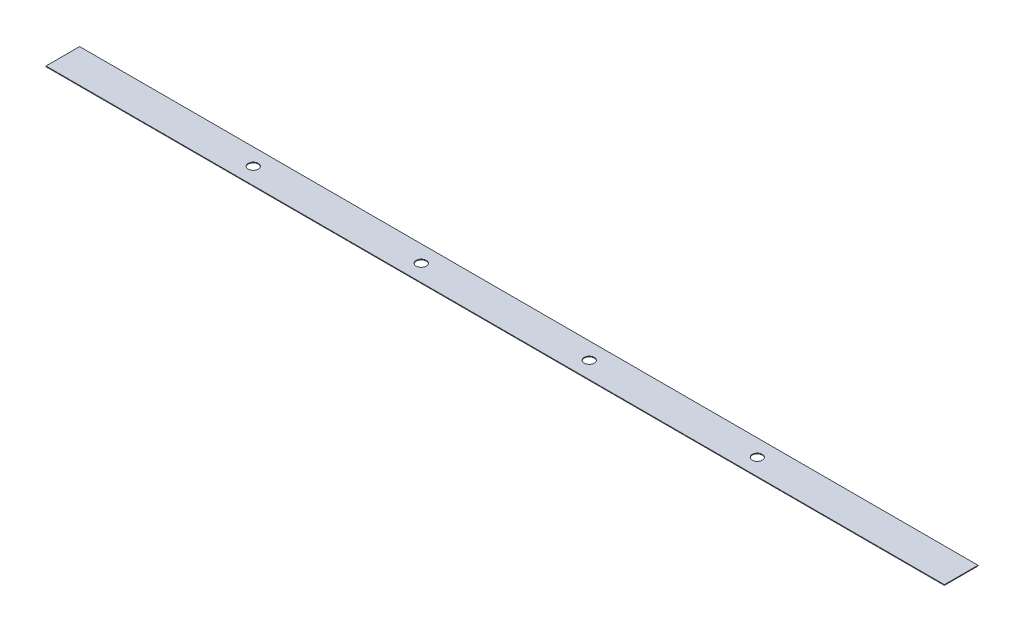
SolidWorks part; units mm, degrees
material "45"
ref_plane "Front Plane" through (0, 0, 0) normal (0, 0, 1) x (1, 0, 0)
ref_plane "Top Plane" through (0, 0, 0) normal (0, 1, 0) x (1, 0, 0)
ref_plane "Right Plane" through (0, 0, 0) normal (1, 0, 0) x (0, 0, -1)
sketch "Sketch1" plane through (0, 0, 0) normal (0, 1, 0) x (1, 0, 0)
  line L1 (-8020, 300) -> (8020, 300)
  line L2 (-8020, 300) -> (-8020, -300)
  line L3 (-8020, -300) -> (8020, -300)
  line L4 (8020, 300) -> (8020, -300)
  line L5 (-8020, 300) -> (8020, -300) construction
  line L6 (-8020, -300) -> (8020, 300) construction
  point P0 (0, 0)
  dimension "D1" = 600
  dimension "D2" = 16040
extrude "Boss-Extrude1" add sketch "Sketch1" along normal blind 12
sketch "Sketch2" plane through (0, 12, 0) normal (0, 1, 0) x (1, 0, 0)
  circle A0 centre (-4620, 0) radius 90
  dimension "D1" = 180
extrude "Cut-Extrude1" cut sketch "Sketch2" against normal through all
pattern_linear "LPattern1" count 4 spacing 3000 along (1, 0, 0) of "Cut-Extrude1"
